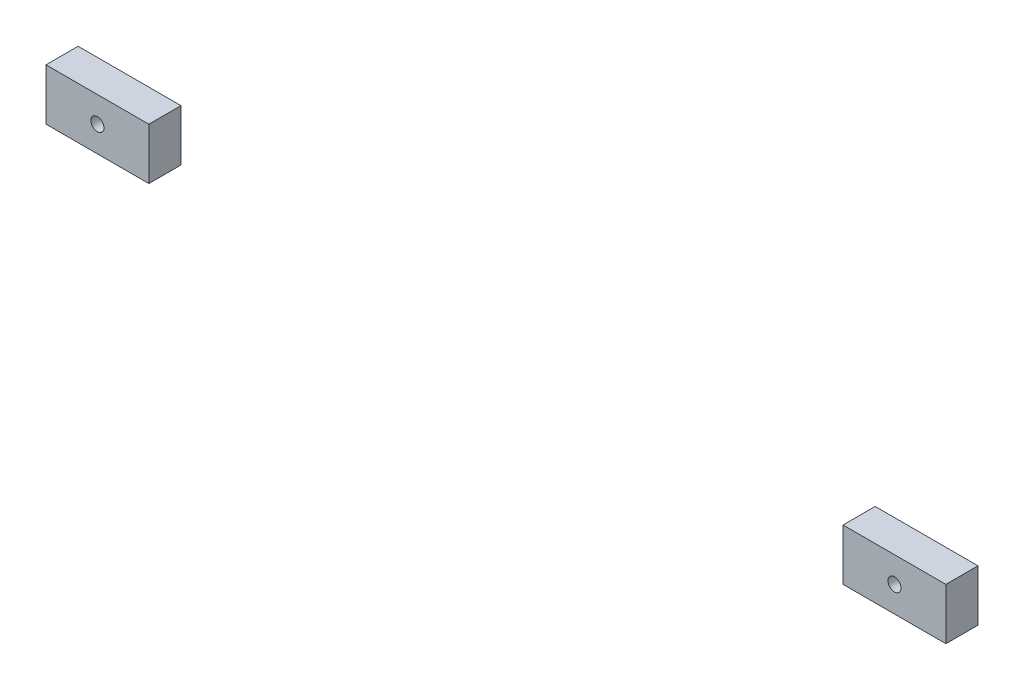
from build123d import *

# Parameters (mm, degrees)
SKETCH1_W                   = 80
SKETCH1_H                   = 40
BOSS_EXTRUDE1_DEPTH         = 25
BOSS_EXTRUDE1_2_DEPTH       = 25
SKETCH3_W                   = 5.1
SKETCH3_H                   = 25
M12_TAPPED_HOLE1_AT_2_COUNT = 2
M12_TAPPED_HOLE1_AT_2_PITCH = 620


with BuildPart() as part:
    # Sketch1 → Boss-Extrude1 (new body)
    with BuildSketch(Plane.XY):
        with Locations((40, -20)):
            Rectangle(SKETCH1_W, SKETCH1_H)
    extrude(amount=BOSS_EXTRUDE1_DEPTH)

    # Sketch3 → M12 Tapped Hole1 (revolve, cut)
    with BuildSketch(Plane(origin=(40, -20, 25), x_dir=(0, -1, 0), z_dir=(1, 0, 0))):
        with Locations((2.55, 12.5)):
            Rectangle(SKETCH3_W, SKETCH3_H)
    m12_tapped_hole1 = revolve(axis=Axis((40, -20, 31.35), (0, 0, -1)), mode=Mode.SUBTRACT)


with BuildPart() as body_2:
    # Sketch1 → Boss-Extrude1 2 (new body)
    with BuildSketch(Plane.XY):
        with Locations((660, -20)):
            Rectangle(SKETCH1_W, SKETCH1_H)
    extrude(amount=BOSS_EXTRUDE1_2_DEPTH)

    # M12 Tapped Hole1 at 2: M12 Tapped Hole1 ×2
    with Locations(*[(i * M12_TAPPED_HOLE1_AT_2_PITCH, 0, 0) for i in range(1, M12_TAPPED_HOLE1_AT_2_COUNT)]):
        add(m12_tapped_hole1, mode=Mode.SUBTRACT)


solid = Compound([part.part, body_2.part])
